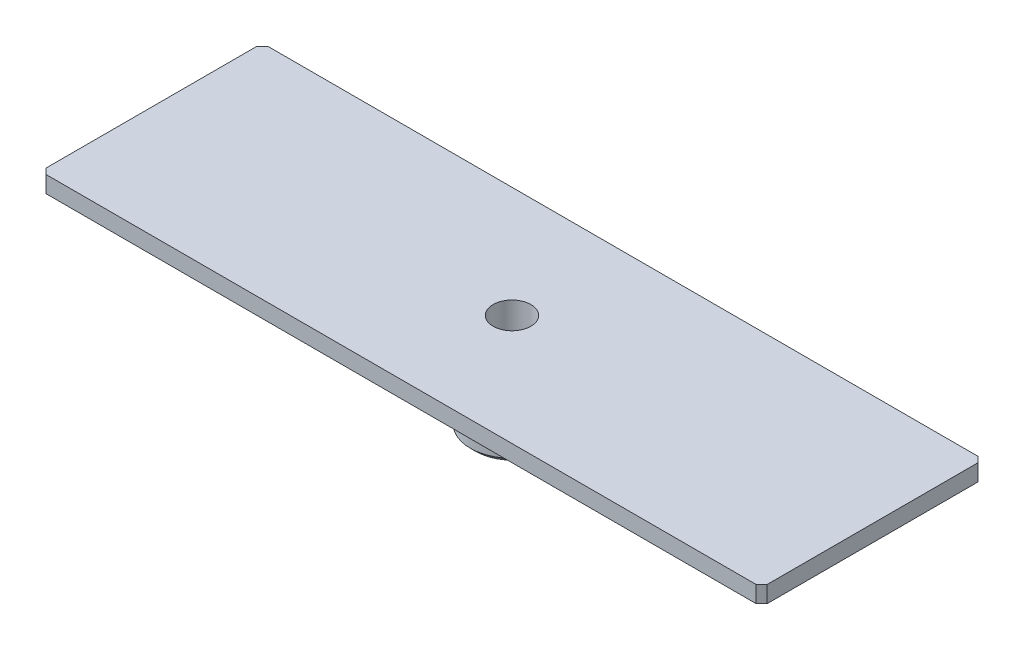
from build123d import *

# Parameters (mm, degrees)
SKETCH1_R             = 7.5
BOSS_EXTRUDE1_DEPTH   = 15
SKETCH2_W             = 130
SKETCH2_H             = 40
BOSS_EXTRUDE2_DEPTH   = 3
M8_TAPPED_HOLE1_D     = 6.8
M8_TAPPED_HOLE1_DEPTH = 19.75
M8_TAPPED_HOLE1_TIP   = 2.042926105
CHAMFER1_SIZE         = 1


with BuildPart() as part:
    # Sketch1 → Boss-Extrude1 (new body)
    with BuildSketch(Plane(origin=(0, 0, 0), x_dir=(1, 0, 0), z_dir=(0, 1, 0))):
        with Locations(Location((0, 0, 0), (0, 0, 270))):
            Circle(SKETCH1_R)
    extrude(amount=BOSS_EXTRUDE1_DEPTH)

    # Sketch2 → Boss-Extrude2 (add)
    with BuildSketch(Plane(origin=(0, 15, 0), x_dir=(1, 0, 0), z_dir=(0, 1, 0))):
        Rectangle(SKETCH2_W, SKETCH2_H)
    extrude(amount=BOSS_EXTRUDE2_DEPTH)

    # M8 Tapped Hole1
    with Locations(Plane(origin=(0, 0, 0), x_dir=(-1, 0, 0), z_dir=(0, -1, 0))):
        with Locations((0, 0)):
            Hole(M8_TAPPED_HOLE1_D / 2, depth=M8_TAPPED_HOLE1_DEPTH)
            with Locations((0, 0, -(M8_TAPPED_HOLE1_DEPTH + M8_TAPPED_HOLE1_TIP / 2))):  # 118° drill point
                Cone(0, M8_TAPPED_HOLE1_D / 2, M8_TAPPED_HOLE1_TIP, mode=Mode.SUBTRACT)

    # Chamfer1
    chamfer1_edges = [part.edges().sort_by_distance(p)[0] for p in [
        (0, 0, -7.5),
        (0, 15, -7.5),
        (65, 16.5, 20),
        (65, 16.5, -20),
        (-65, 16.5, -20),
        (-65, 16.5, 20),
    ]]
    chamfer(chamfer1_edges, length=CHAMFER1_SIZE)


solid = part.part
